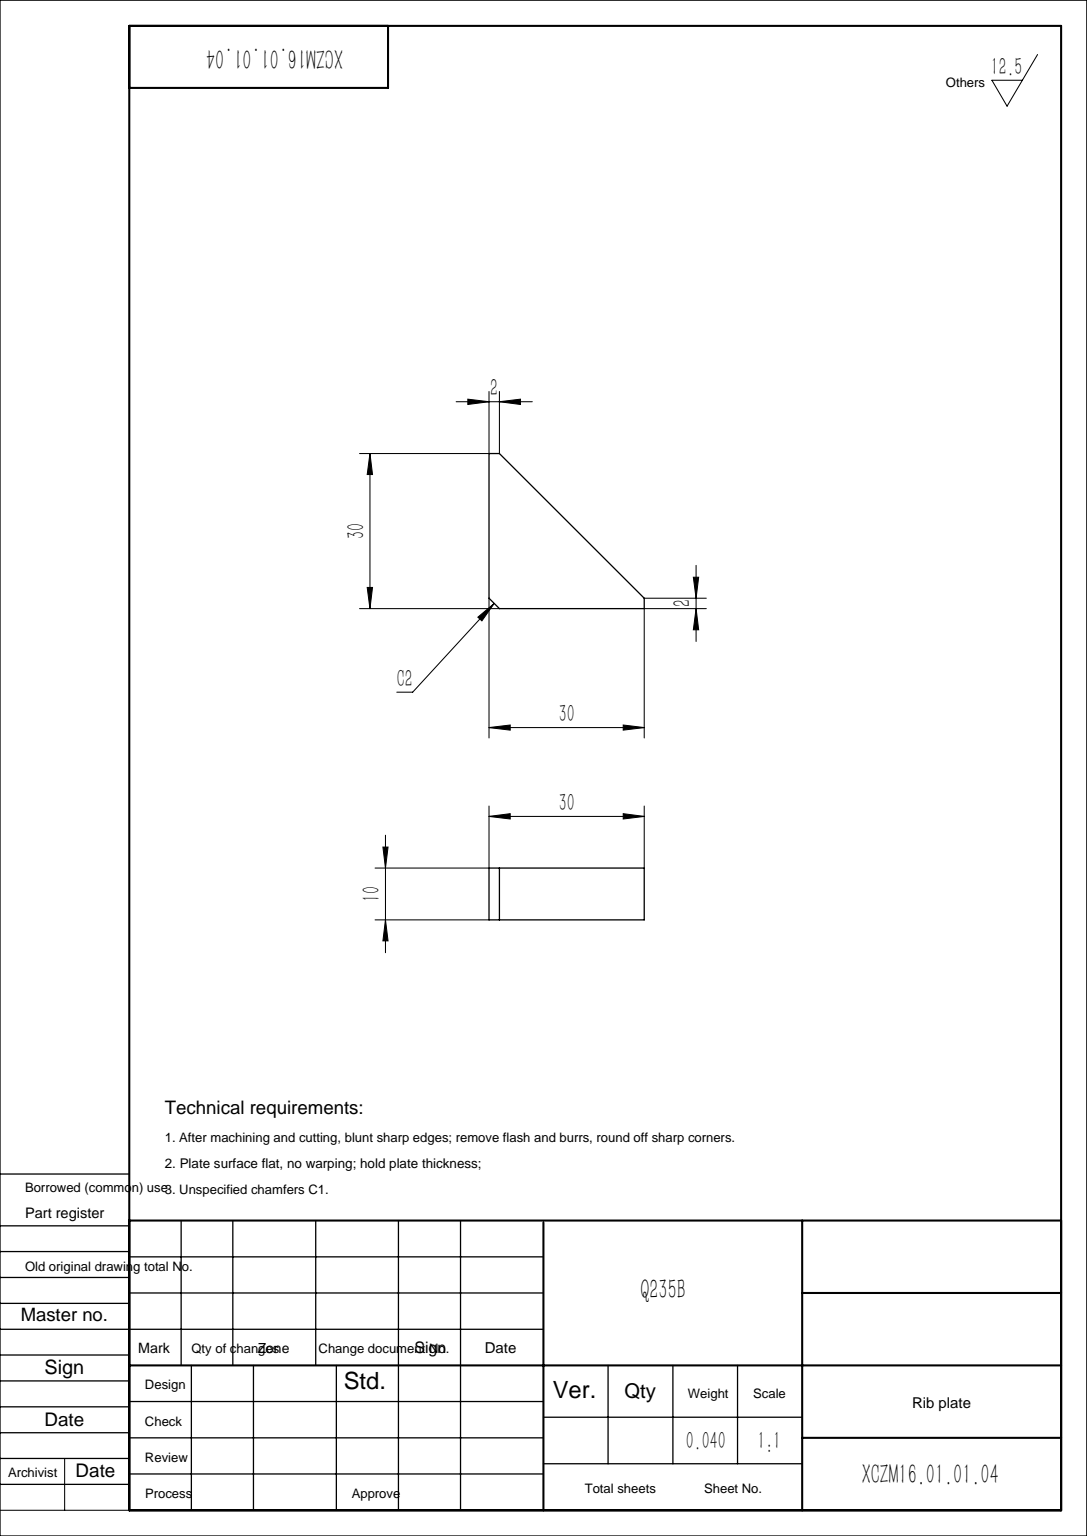
from build123d import *

# Parameters (mm, degrees)
EXTRUDE_1_DEPTH = 10
CHAMFER_1_SIZE  = 2


with BuildPart() as part:
    # 草图1 → 凸台-拉伸1 (new body)
    with BuildSketch(Plane.XY):
        Polygon((0, 30), (0, 0), (30, 0), (30, 2), (2, 30), align=None)
    extrude(amount=EXTRUDE_1_DEPTH)

    # 倒角1
    chamfer_1_edges = [part.edges().sort_by_distance(p)[0] for p in [
        (0, 0, 5),
    ]]
    chamfer(chamfer_1_edges, length=CHAMFER_1_SIZE)


solid = part.part
